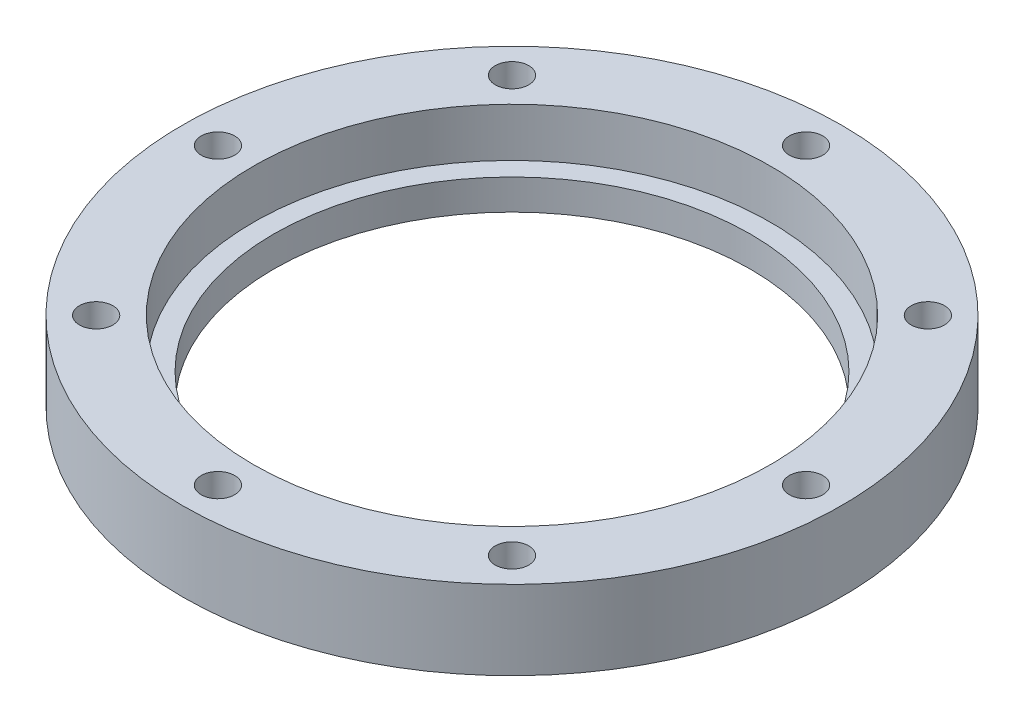
SolidWorks part; units mm, degrees
material "6061 合金"
ref_plane "前视基准面" through (0, 0, 0) normal (0, 0, 1) x (1, 0, 0)
ref_plane "上视基准面" through (0, 0, 0) normal (0, 1, 0) x (1, 0, 0)
ref_plane "右视基准面" through (0, 0, 0) normal (1, 0, 0) x (0, 0, -1)
sketch "草图1" plane through (0, 0, 0) normal (0, 1, 0) x (1, 0, 0)
  circle A0 centre (0, 0) radius 23.5
  circle A1 centre (0, 0) radius 32.5
  dimension "D1" = 47
  dimension "D2" = 65
extrude "凸台-拉伸1" add sketch "草图1" along normal blind 3
sketch "草图2" plane through (0, 3, 0) normal (0, 1, 0) x (1, 0, 0)
  circle A0 centre (0, 0) radius 25.5
  circle A1 centre (0, 0) radius 32.5 construction
  circle A2 centre (0, 0) radius 32.5
  dimension "D1" = 51
extrude "凸台-拉伸2" add sketch "草图2" along normal blind 4.8
sketch "草图3" plane through (0, 7.8, 0) normal (0, 1, 0) x (1, 0, 0)
  point P0 (0, 29)
  point P1 (20.5061, 20.5061)
  point P5 (29, 0)
  point P6 (20.5061, -20.5061)
  point P7 (0, -29)
  point P8 (-20.5061, -20.5061)
  point P9 (-29, 0)
  point P10 (-20.5061, 20.5061)
  point P11 (0, 0)
  dimension "D1" = 29
  dimension "D2" = 8
hole_wizard "M4 螺纹孔1" positions "草图3" profile "草图4" tap size "M4" standard "GB" end condition through all
sketch "草图4" plane through (0, 7.8, -29) normal (1, 0, 0) x (0, 0, 1)
  line L0 (0, 0) -> (0, 7.8)
  line L1 (0, 7.8) -> (1.65, 7.8)
  line L2 (1.65, 7.8) -> (1.65, 0)
  line L5 (1.65, 0) -> (0, 0)
  line L11 (0, -6.35) -> (0, 107.95) construction
  dimension "通孔螺纹孔钻头直径" = 3.3
  dimension "通孔螺纹孔钻头深度" = 7.8
cosmetic thread "孔螺纹线1" parameters "D2"=4
cosmetic thread "孔螺纹线2" parameters "D2"=4
cosmetic thread "孔螺纹线3" parameters "D2"=4
cosmetic thread "孔螺纹线4" parameters "D2"=4
cosmetic thread "孔螺纹线5" parameters "D2"=4
cosmetic thread "孔螺纹线6" parameters "D2"=4
cosmetic thread "孔螺纹线7" parameters "D2"=4
cosmetic thread "孔螺纹线8" parameters "D2"=4
